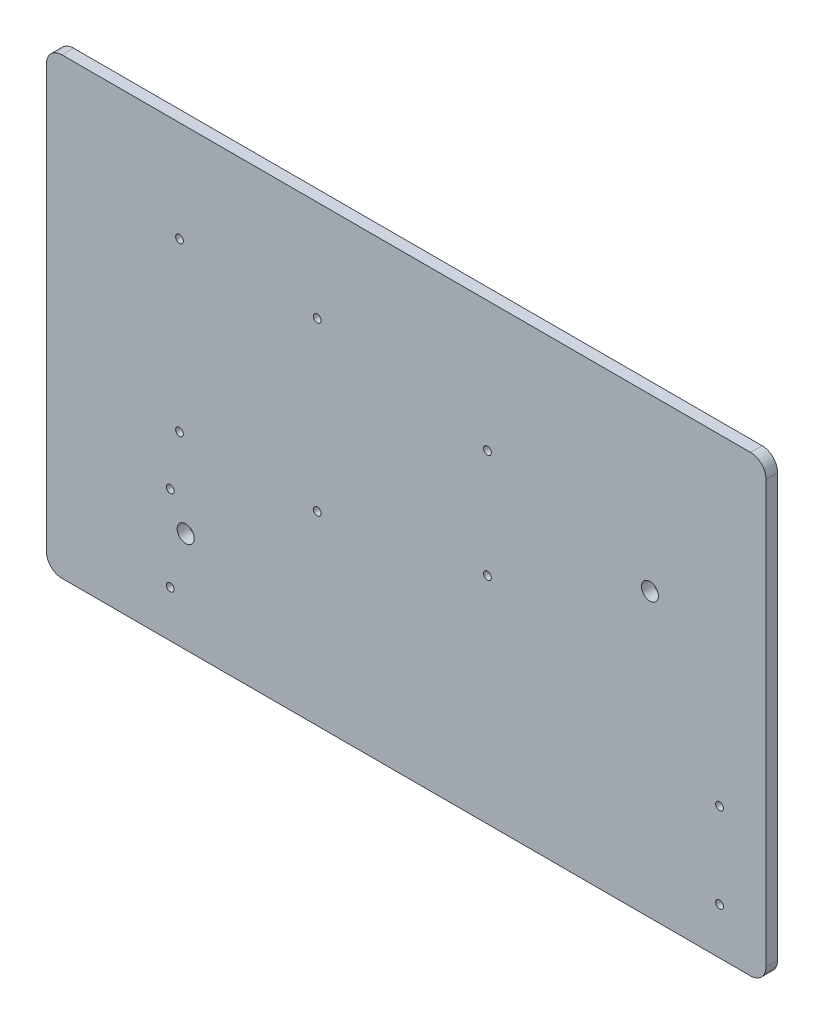
from build123d import *

# Parameters (mm, degrees)
SKETCH_1_R           = 5
SKETCH_1_R_2         = 11
BOSS_EXTRUDE_1_DEPTH = 15


with BuildPart() as part:
    # Sketch 1 → Boss-Extrude 1 (new body)
    with BuildSketch(Plane.XY):
        with BuildLine():
            Line((-465, -273), (-465, 273))
            ThreePointArc((-465, 273), (-459.142135624, 287.142135624), (-445, 293))
            Line((-445, 293), (445, 293))
            ThreePointArc((445, 293), (459.142135624, 287.142135624), (465, 273))
            Line((465, 273), (465, -273))
            ThreePointArc((465, -273), (459.142135624, -287.142135624), (445, -293))
            Line((445, -293), (-445, -293))
            ThreePointArc((-445, -293), (-459.142135624, -287.142135624), (-465, -273))
        make_face()
        with Locations((-115, 163)):
            Circle(SKETCH_1_R, mode=Mode.SUBTRACT)
        with Locations((-293, 163)):
            Circle(SKETCH_1_R, mode=Mode.SUBTRACT)
        with Locations(Location((-293, -53, 0), (0, 0, 180))):
            Circle(SKETCH_1_R, mode=Mode.SUBTRACT)
        with Locations((105, -15)):
            Circle(SKETCH_1_R, mode=Mode.SUBTRACT)
        with Locations(Location((-115, -53, 0), (0, 0, 180))):
            Circle(SKETCH_1_R, mode=Mode.SUBTRACT)
        with Locations(Location((105, 125, 0), (0, 0, 180))):
            Circle(SKETCH_1_R, mode=Mode.SUBTRACT)
        with Locations((-305, -123)):
            Circle(SKETCH_1_R, mode=Mode.SUBTRACT)
        with Locations(Location((-305, -233, 0), (0, 0, 180))):
            Circle(SKETCH_1_R, mode=Mode.SUBTRACT)
        with Locations((405, -233)):
            Circle(SKETCH_1_R, mode=Mode.SUBTRACT)
        with Locations(Location((405, -123, 0), (0, 0, 180))):
            Circle(SKETCH_1_R, mode=Mode.SUBTRACT)
        with Locations((315, 72.5)):
            Circle(SKETCH_1_R_2, mode=Mode.SUBTRACT)
        with Locations((-285, -163)):
            Circle(SKETCH_1_R_2, mode=Mode.SUBTRACT)
    extrude(amount=BOSS_EXTRUDE_1_DEPTH)


solid = part.part
